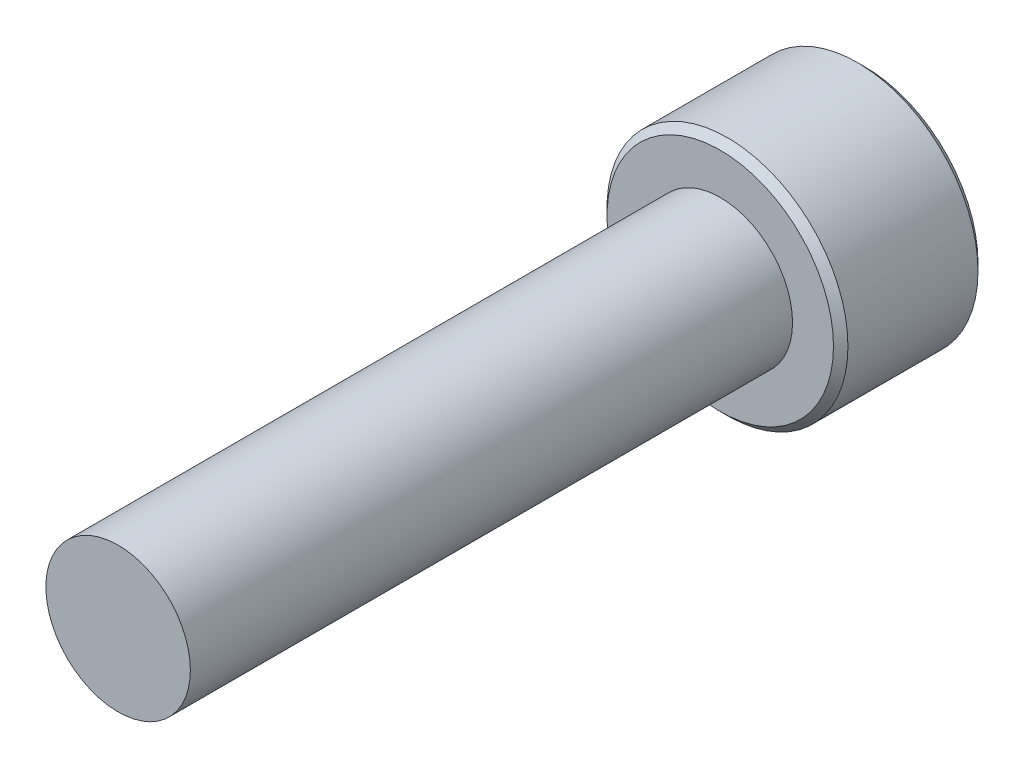
from build123d import *

# Parameters (mm, degrees)
SKETCH1_R           = 5
BOSS_EXTRUDE1_DEPTH = 6
SKETCH2_R           = 3
BOSS_EXTRUDE2_DEPTH = 25
CHAMFER1_SIZE       = 0.3
CUT_EXTRUDE1_DEPTH  = 3


with BuildPart() as part:
    # Sketch1 → Boss-Extrude1 (new body)
    with BuildSketch(Plane.XY):
        Circle(SKETCH1_R)
    extrude(amount=BOSS_EXTRUDE1_DEPTH)

    # Sketch2 → Boss-Extrude2 (add)
    with BuildSketch(Plane.XY.offset(6)):
        Circle(SKETCH2_R)
    extrude(amount=BOSS_EXTRUDE2_DEPTH)

    # Chamfer1
    chamfer1_edges = [part.edges().sort_by_distance(p)[0] for p in [
        (-5, 0, 0),
        (-5, 0, 6),
    ]]
    chamfer(chamfer1_edges, length=CHAMFER1_SIZE)

    # Sketch3 → Cut-Extrude1 (cut)
    with BuildSketch(Plane(origin=(0, 0, 0), x_dir=(-1, 0, 0), z_dir=(0, 0, -1))):
        Polygon((0, 2.42932406), (-2.10385635, 1.21466203), (-2.10385635, -1.21466203), (0, -2.42932406), (2.10385635, -1.21466203), (2.10385635, 1.21466203), align=None)
    extrude(amount=-CUT_EXTRUDE1_DEPTH, mode=Mode.SUBTRACT)


solid = part.part
